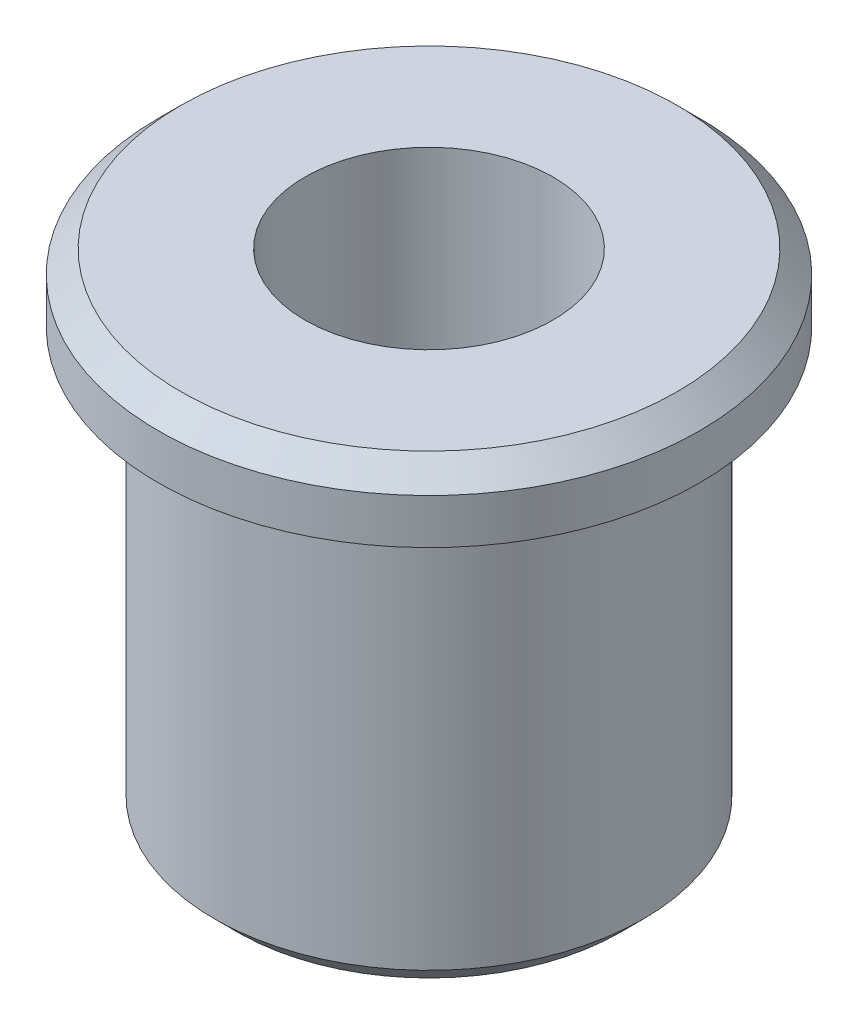
from build123d import *

# Parameters (mm, degrees)
CUT_EXTRUDE_1_DEPTH      = 28.784887979
CUT_EXTRUDE_1_DEPTH_BACK = 28.784887979
SKETCH_2_R               = 5.5
CHAMFER_1_SIZE           = 1
CHAMFER_2_SIZE           = 1


with BuildPart() as part:
    # 草图1 → 旋转1 (revolve)
    with BuildSketch(Plane.XY):
        Polygon((0, 0), (0, 22), (12, 22), (12, 19), (9.5, 19), (9.5, 0), align=None)
    revolve(axis=Axis((0, 0, 0), (0, 1, 0)))

    # 草图2 → 切除-拉伸1 (cut, two sides: drawn at the far end of the back side and taken through both)
    with BuildSketch(Plane.XZ.offset(-CUT_EXTRUDE_1_DEPTH_BACK)):
        with Locations(Location((0, 0, 0), (0, 0, 270))):
            Circle(SKETCH_2_R)
    extrude(amount=CUT_EXTRUDE_1_DEPTH + CUT_EXTRUDE_1_DEPTH_BACK, mode=Mode.SUBTRACT)

    # 倒角1
    chamfer_1_edges = [part.edges().sort_by_distance(p)[0] for p in [
        (-12, 22, 0),
    ]]
    chamfer(chamfer_1_edges, length=CHAMFER_1_SIZE)

    # 倒角2
    chamfer_2_edges = [part.edges().sort_by_distance(p)[0] for p in [
        (-9.5, 0, 0),
    ]]
    chamfer(chamfer_2_edges, length=CHAMFER_2_SIZE)


solid = part.part
